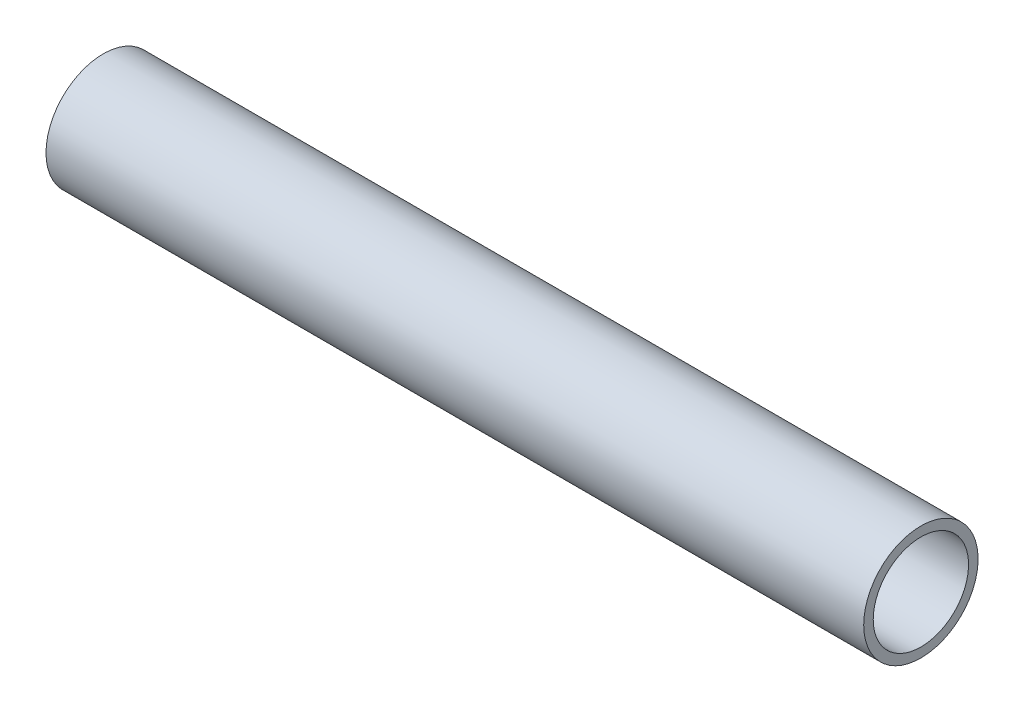
from build123d import *

# Parameters (mm, degrees)
SWEEP_1_PROFILE_R   = 6
SWEEP_1_PROFILE_R_2 = 5


with BuildPart() as part:
    # 扫描-薄件1: sweep along a curve in space
    with BuildLine() as sweep_1_path:
        Line((860.166218058, 1814.095116422, 422.912562332), (774.409502338, 1814.095116422, 422.912562332))
    # 扫描-薄件1 profile (on start of the path) → 扫描-薄件1 (sweep)
    with BuildSketch(Plane(origin=(860.166218058, 1814.095116422, 422.912562332), x_dir=(0, 0, -1), z_dir=(-1, 0, 0))):
        Circle(SWEEP_1_PROFILE_R)
        Circle(SWEEP_1_PROFILE_R_2, mode=Mode.SUBTRACT)
    sweep(path=sweep_1_path.line)


solid = part.part
